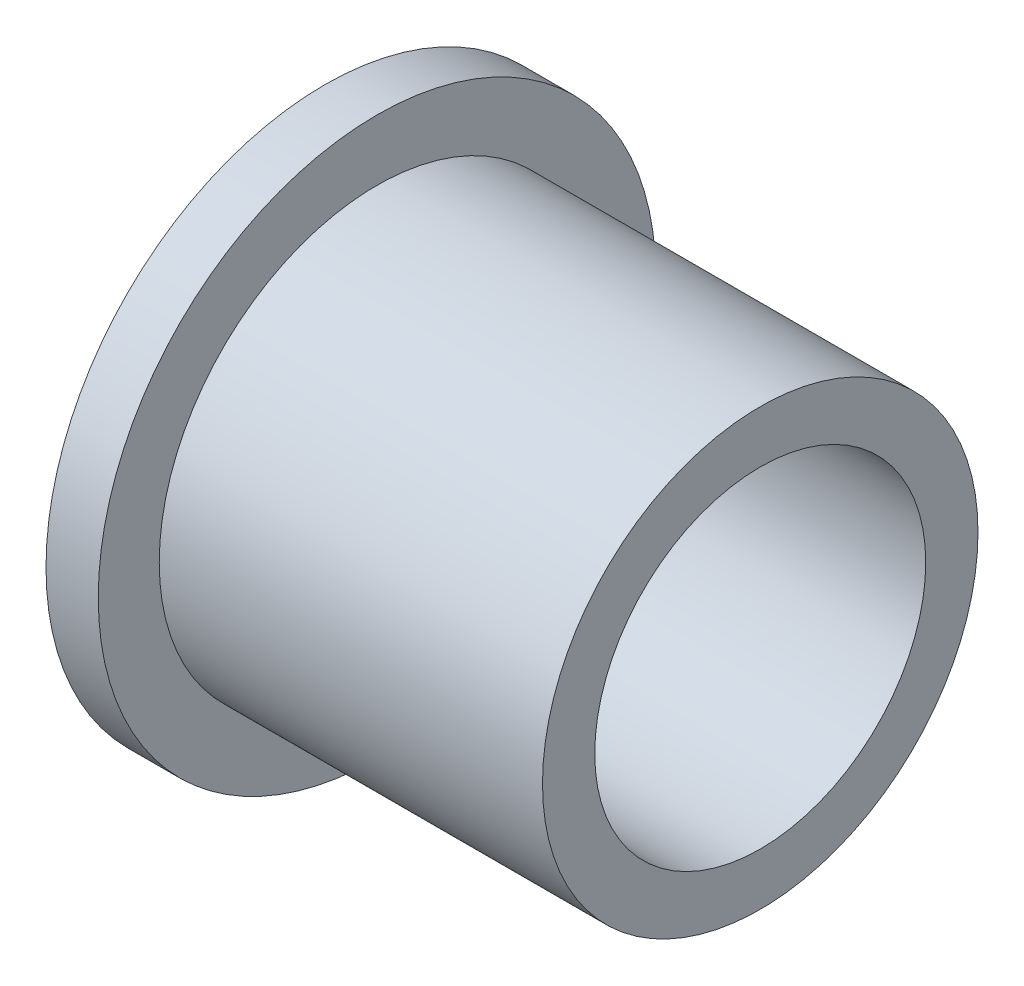
from build123d import *


with BuildPart() as part:
    # Sketch1 → Revolve1 (revolve)
    with BuildSketch(Plane.XY, mode=Mode.PRIVATE) as revolve1_sk:
        Polygon((0, 241.3), (0, 406.4), (76.2, 406.4), (76.2, 317.5), (635, 317.5), (635, 241.3), align=None)
    revolve(revolve1_sk.sketch.rotate(Axis((0, 0, 0), (1, 0, 0)), 90), axis=Axis((0, 0, 0), (1, 0, 0)))


solid = part.part
